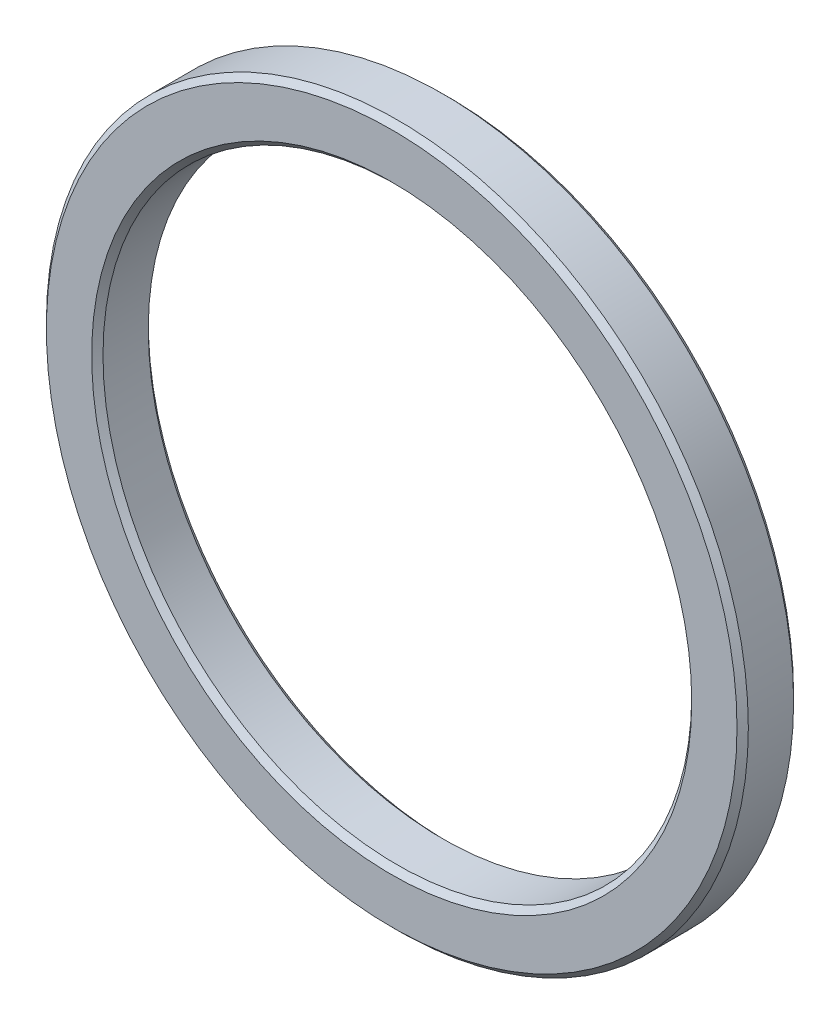
SolidWorks part; units mm, degrees
ref_plane "Front Plane" through (0, 0, 0) normal (0, 0, 1) x (1, 0, 0)
ref_plane "Top Plane" through (0, 0, 0) normal (0, 1, 0) x (1, 0, 0)
ref_plane "Right Plane" through (0, 0, 0) normal (1, 0, 0) x (0, 0, -1)
sketch "Sketch1" plane through (0, 0, 0) normal (0, 0, 1) x (1, 0, 0)
  circle A0 centre (0, 0) radius 31
  circle A1 centre (0, 0) radius 26
extrude "Boss-Extrude1" add sketch "Sketch1" along normal blind 5
chamfer "Chamfer1" distance 0.5 angle 45 4 edges at (26, 0, 0) (31, 0, 0) (26, 0, 5) (31, 0, 5)
